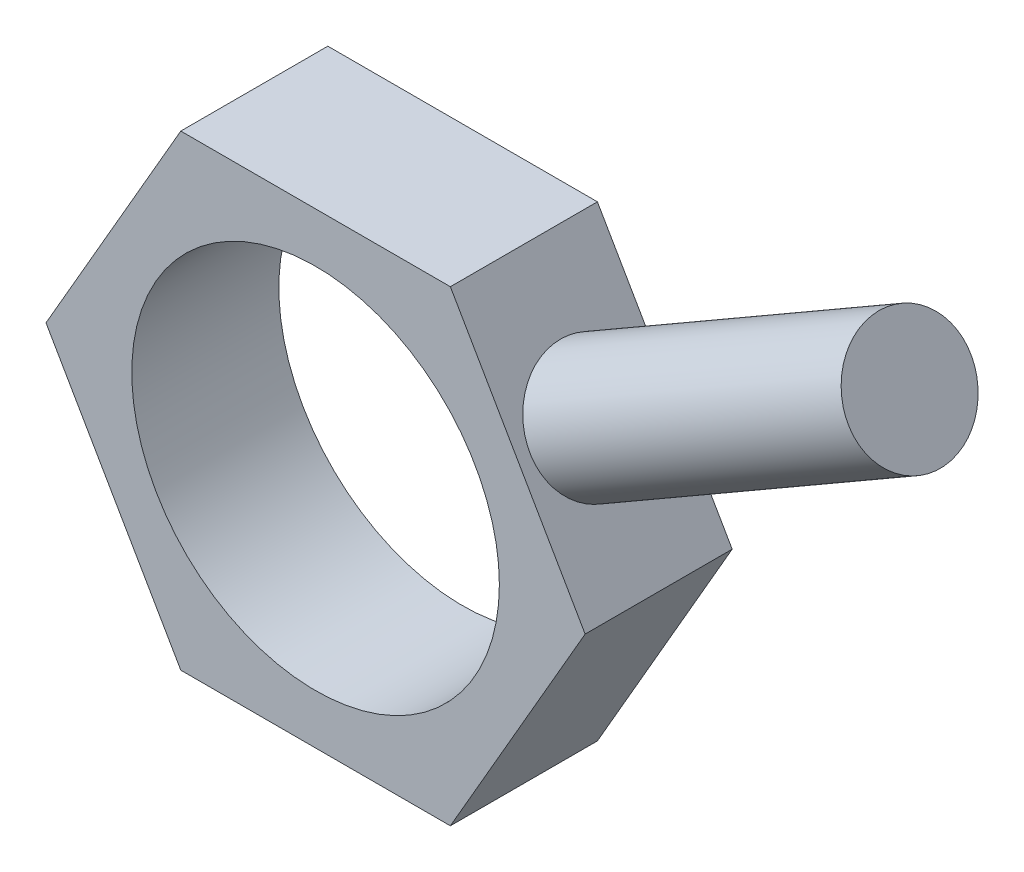
from build123d import *

# Parameters (mm, degrees)
SKETCH1_R           = 7.5
BOSS_EXTRUDE1_DEPTH = 6
SKETCH2_R           = 2.5
BOSS_EXTRUDE2_DEPTH = 15


with BuildPart() as part:
    # Sketch1 → Boss-Extrude1 (new body)
    with BuildSketch(Plane.XY):
        Polygon((-5.5, 9.526279442), (-11, 0), (-5.5, -9.526279442), (5.5, -9.526279442), (11, 0), (5.5, 9.526279442), align=None)
        Circle(SKETCH1_R, mode=Mode.SUBTRACT)
    extrude(amount=BOSS_EXTRUDE1_DEPTH)

    # Sketch2 → Boss-Extrude2 (add)
    with BuildSketch(Plane(origin=(8.25, 4.763139721, 0), x_dir=(0, 0, -1), z_dir=(0.8660254037844389, 0.49999999999999983, 0))):
        with Locations(Location((-3, 0, 0), (0, 0, 90))):
            Circle(SKETCH2_R)
    extrude(amount=BOSS_EXTRUDE2_DEPTH)


solid = part.part
